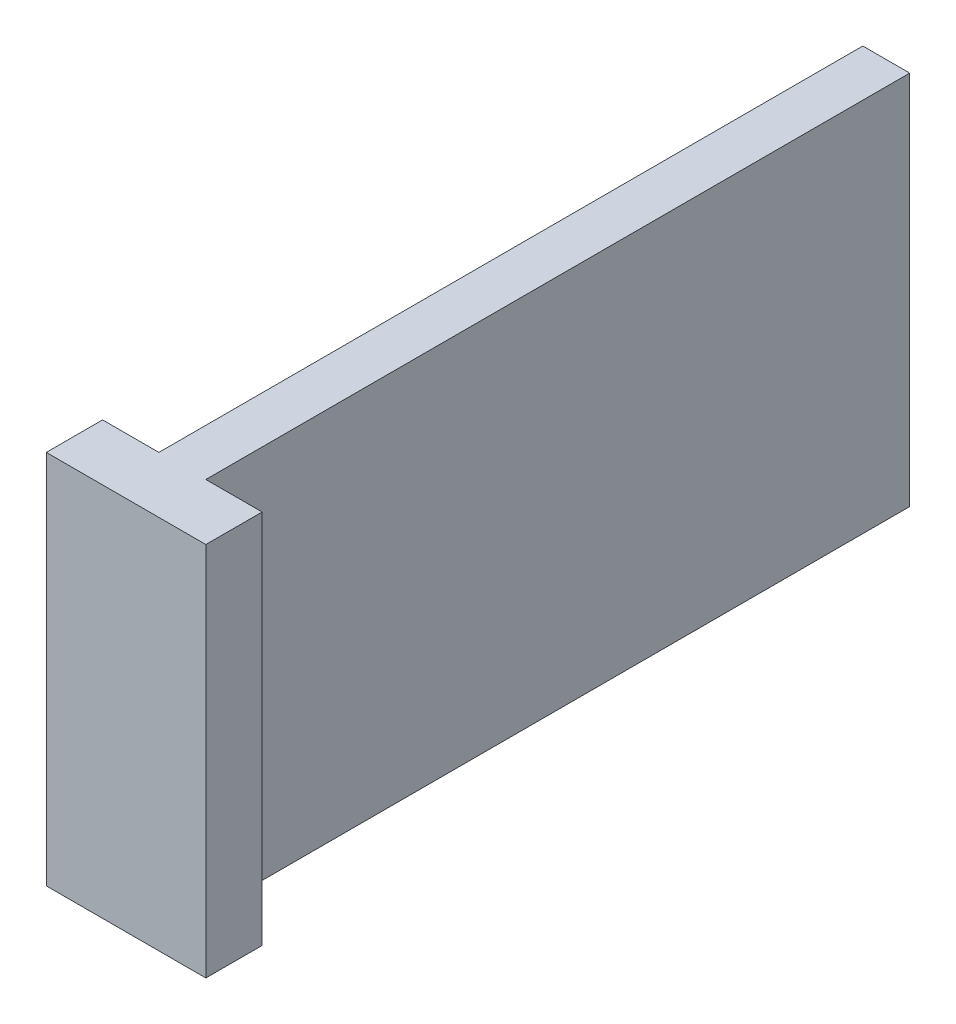
SolidWorks part; units mm, degrees
ref_plane "前视基准面" through (0, 0, 0) normal (0, 0, 1) x (1, 0, 0)
ref_plane "上视基准面" through (0, 0, 0) normal (0, 1, 0) x (1, 0, 0)
ref_plane "右视基准面" through (0, 0, 0) normal (1, 0, 0) x (0, 0, -1)
sketch "草图1" plane through (0, 0, 0) normal (1, 0, 0) x (0, 0, -1)
  line L1 (-75, -40) -> (75, -40)
  line L2 (-75, -40) -> (-75, 40)
  line L3 (-75, 40) -> (75, 40)
  line L4 (75, -40) -> (75, 40)
  line L5 (-75, -40) -> (75, 40) construction
  line L6 (-75, 40) -> (75, -40) construction
  point P0 (0, 0)
  dimension "D1" = 80
  dimension "D2" = 150
extrude "凸台-拉伸1" add sketch "草图1" along normal mid plane 10
sketch "草图2" plane through (0, 0, 75) normal (0, 0, 1) x (1, 0, 0)
  line L0 (-5, 40) -> (-5, -40) construction
  line L1 (-5, -40) -> (17, -40)
  line L2 (-5, -40) -> (-5, 40)
  line L3 (-5, 40) -> (17, 40)
  line L4 (17, -40) -> (17, 40)
  line L5 (5, 40) -> (-5, 40) construction
  line L6 (5, 40) -> (5, -40) construction
  dimension "D1" = 12
extrude "凸台-拉伸2" add sketch "草图2" along normal blind 12
mirror "镜向1" about plane through (0, 0, 0) normal (1, 0, 0) of "凸台-拉伸2"
